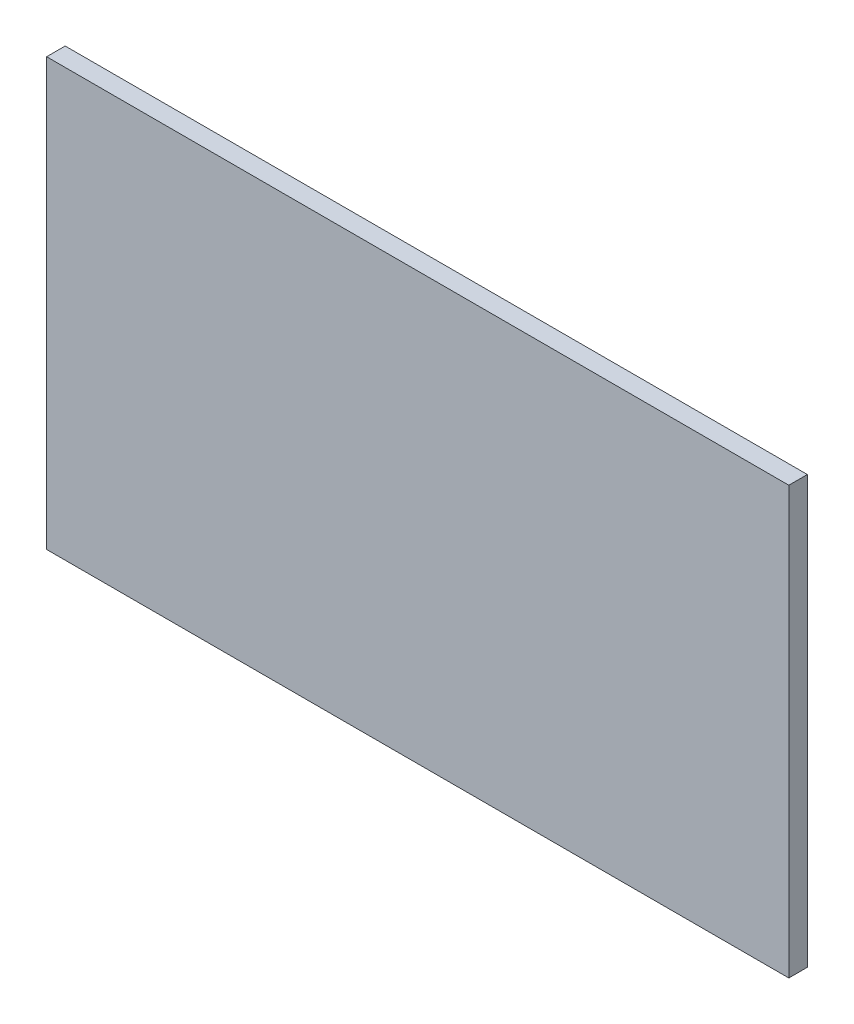
SolidWorks part; units mm, degrees
ref_plane "Front Plane" through (0, 0, 0) normal (0, 0, 1) x (1, 0, 0)
ref_plane "Top Plane" through (0, 0, 0) normal (0, 1, 0) x (1, 0, 0)
ref_plane "Right Plane" through (0, 0, 0) normal (1, 0, 0) x (0, 0, -1)
sketch "Sketch1" plane through (0, 0, 0) normal (0, 0, 1) x (1, 0, 0)
  line L2 (200, -115) -> (-200, -115)
  line L3 (200, -115) -> (200, 115)
  line L4 (200, 115) -> (-200, 115)
  line L5 (-200, -115) -> (-200, 115)
  line L6 (200, -115) -> (-200, 115) construction
  line L7 (200, 115) -> (-200, -115) construction
  point P2 (0, 0)
  dimension "D1" = 400
  dimension "D2" = 230
extrude "Boss-Extrude1" add sketch "Sketch1" along normal blind 10
